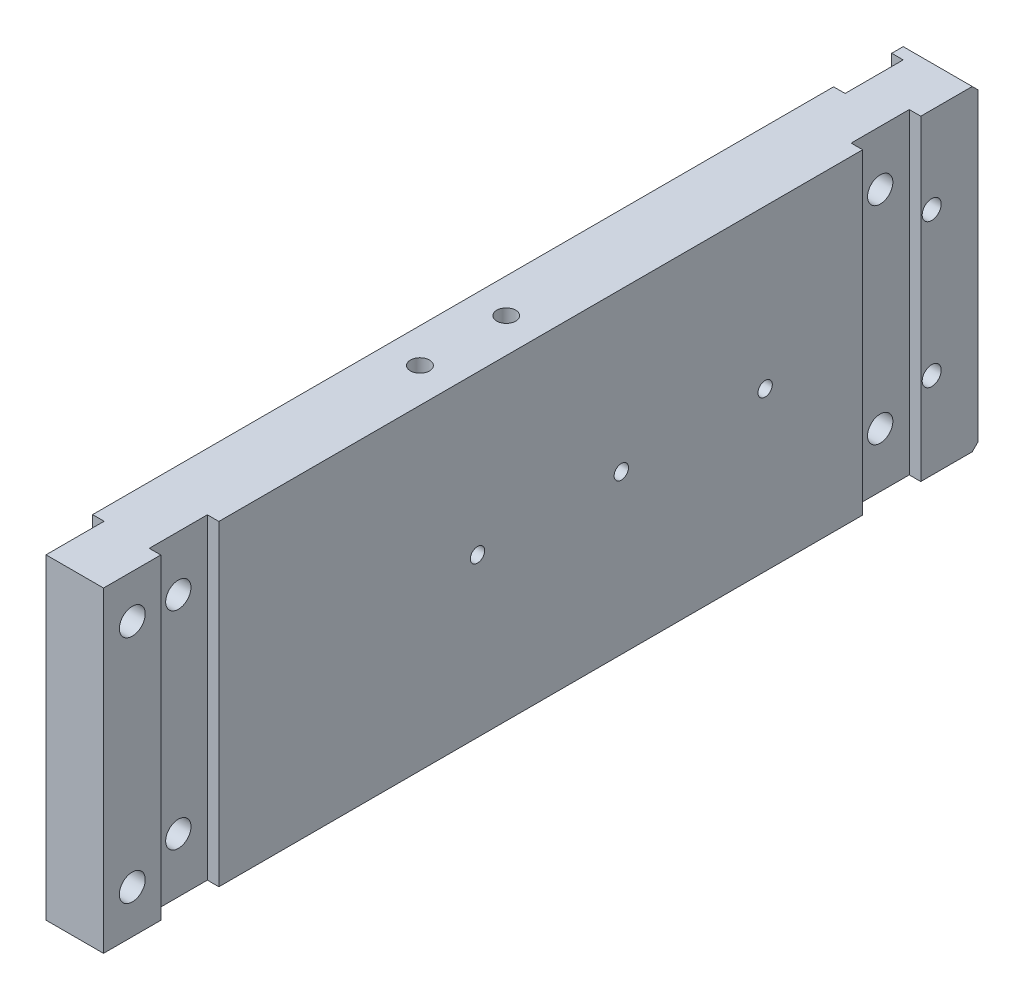
from build123d import *

# Parameters (mm, degrees)
SKETCH_1_W                  = 152
SKETCH_1_H                  = 55
EXTRUDE_1_DEPTH             = 12
SKETCH_2_W                  = 10.1
SKETCH_2_H                  = 67.741828953
CUT_EXTRUDE_1_DEPTH         = 2
SKETCH_3_W                  = 81
SKETCH_3_H                  = 12.05
CUT_EXTRUDE_2_DEPTH         = 1.5
SKETCH_4_R                  = 2
CUT_EXTRUDE_3_DEPTH         = 1.5
SKETCH_5_W                  = 2
SKETCH_5_H                  = 10.1
CUT_EXTRUDE_4_DEPTH         = 110
SKETCH_7_W                  = 4
SKETCH_7_H                  = 10.1
CUT_EXTRUDE_5_DEPTH         = 120
CHAMFER_1_SIZE              = 1
HOLE_WIZARD_M4_1_AT_2_COUNT = 2
HOLE_WIZARD_M4_1_AT_2_PITCH = 15
HOLE_WIZARD_5_0_5_2_D       = 5
HOLE_WIZARD_5_0_5_2_DEPTH   = 6
HOLE_WIZARD_5_0_5_2_TIP     = 1.502151548
HOLE_WIZARD_1_D             = 4.4
HOLE_WIZARD_1_CBORE_D       = 8
HOLE_WIZARD_1_CBORE_DEPTH   = 6
HOLE_WIZARD_M3_1_D          = 2.5
HOLE_WIZARD_M4_2_D          = 3.3
HOLE_WIZARD_M4_2_DEPTH      = 11.5
HOLE_WIZARD_M4_2_TIP        = 0.991420021
HOLE_WIZARD_M4_3_D          = 3.3
SKETCH_30_R                 = 2.25
CUT_EXTRUDE_6_DEPTH         = 25


with BuildPart() as part:
    # 草图1 → 凸台-拉伸1 (new body)
    with BuildSketch(Plane(origin=(0, 0, 0), x_dir=(0, 0, -1), z_dir=(1, 0, 0))):
        Rectangle(SKETCH_1_W, SKETCH_1_H)
    extrude(amount=EXTRUDE_1_DEPTH)

    # 草图2 → 切除-拉伸1 (cut)
    with BuildSketch(Plane(origin=(12, 0, 0), x_dir=(0, 0, -1), z_dir=(1, 0, 0))):
        with Locations((-61, -0.529795054)):
            Rectangle(SKETCH_2_W, SKETCH_2_H)
    cut_extrude_1 = extrude(amount=-CUT_EXTRUDE_1_DEPTH, mode=Mode.SUBTRACT)

    # 草图3 → 切除-拉伸2 (cut)
    with BuildSketch(Plane.ZY):
        with Locations((-13.5, 0)):
            Rectangle(SKETCH_3_W, SKETCH_3_H)
    extrude(amount=-CUT_EXTRUDE_2_DEPTH, mode=Mode.SUBTRACT)

    # 草图4 → 切除-拉伸3 (cut)
    with BuildSketch(Plane.ZY):
        with Locations((-54, 6.025)):
            Circle(SKETCH_4_R)
        with Locations((-54, -6.025)):
            Circle(SKETCH_4_R)
        with Locations((27, -6.025)):
            Circle(SKETCH_4_R)
        with Locations((27, 6.025)):
            Circle(SKETCH_4_R)
    extrude(amount=-CUT_EXTRUDE_3_DEPTH, mode=Mode.SUBTRACT)

    # 草图5 → 切除-拉伸4 (cut)
    with BuildSketch(Plane.XZ.offset(27.5)):
        with Locations((1, 70.95)):
            Rectangle(SKETCH_5_W, SKETCH_5_H)
    extrude(amount=-CUT_EXTRUDE_4_DEPTH, mode=Mode.SUBTRACT)

    # 草图7 → 切除-拉伸5 (cut)
    with BuildSketch(Plane(origin=(0, 27.5, 0), x_dir=(1, 0, 0), z_dir=(0, 1, 0))):
        with Locations((0, 67.95)):
            Rectangle(SKETCH_7_W, SKETCH_7_H)
    extrude(amount=-CUT_EXTRUDE_5_DEPTH, mode=Mode.SUBTRACT)

    # 倒角1
    chamfer_1_edges = [part.edges().sort_by_distance(p)[0] for p in [
        (6, -27.5, -76),
        (6, 27.5, -76),
    ]]
    chamfer(chamfer_1_edges, length=CHAMFER_1_SIZE)

    # 草图9 → M4 螺纹孔1 (revolve, cut)
    with BuildSketch(Plane(origin=(6, 27.5, 15), x_dir=(0, 0, 1), z_dir=(1, 0, 0))):
        Polygon((0, 0), (0, 11.091420021), (1.65, 10.1), (1.65, 0), align=None)
    hole_wizard_m4_1 = revolve(axis=Axis((6, 33.85, 15), (0, -1, 0)), mode=Mode.SUBTRACT)

    # M4 螺纹孔1 at 2: M4 螺纹孔1 ×2
    with Locations(*[(0, 0, -i * HOLE_WIZARD_M4_1_AT_2_PITCH) for i in range(1, HOLE_WIZARD_M4_1_AT_2_COUNT)]):
        add(hole_wizard_m4_1, mode=Mode.SUBTRACT)

    # 镜向1: M4 螺纹孔1 across plane
    add(hole_wizard_m4_1.mirror(Plane.ZX), mode=Mode.SUBTRACT)

    # 镜向1 copy 1 sketch → 镜向1 copy 1 (revolve, cut)
    with BuildSketch(Plane(origin=(6, -27.5, 0), x_dir=(0, 0, 1), z_dir=(1, 0, 0))):
        Polygon((0, 0), (0, -11.091420021), (1.65, -10.1), (1.65, 0), align=None)
    revolve(axis=Axis((6, -33.85, 0), (0, -1, 0)), mode=Mode.SUBTRACT)

    # Ø5.0 (5) 直径孔2
    with Locations(Plane.ZY.offset(-2)):
        with Locations((70.9, 12.5), (70.9, -12.5)):
            Hole(HOLE_WIZARD_5_0_5_2_D / 2, depth=HOLE_WIZARD_5_0_5_2_DEPTH)
            with Locations((0, 0, -(HOLE_WIZARD_5_0_5_2_DEPTH + HOLE_WIZARD_5_0_5_2_TIP / 2))):  # 118° drill point
                Cone(0, HOLE_WIZARD_5_0_5_2_D / 2, HOLE_WIZARD_5_0_5_2_TIP, mode=Mode.SUBTRACT)

    # 镜向2: 切除-拉伸1 across plane
    add(cut_extrude_1.mirror(Plane.XY), mode=Mode.SUBTRACT)

    # 打孔尺寸(%根据)内六角圆柱头螺钉的类型1 (through all)
    with Locations(Plane.ZY):
        with Locations((61, -18), (61, 18), (-61, 18), (-61, -18)):
            CounterBoreHole(HOLE_WIZARD_1_D / 2, HOLE_WIZARD_1_CBORE_D / 2, HOLE_WIZARD_1_CBORE_DEPTH)

    # M3 螺纹孔1 (through all)
    with Locations(Plane.ZY):
        with Locations((11, 0), (-14, 0), (-39, 0)):
            Hole(HOLE_WIZARD_M3_1_D / 2)

    # M4 螺纹孔2
    with Locations(Plane(origin=(0, -27.5, 0), x_dir=(-1, 0, 0), z_dir=(0, -1, 0))):
        with Locations((-6, 44.926), (-6, 59.926)):
            Hole(HOLE_WIZARD_M4_2_D / 2, depth=HOLE_WIZARD_M4_2_DEPTH)
            with Locations((0, 0, -(HOLE_WIZARD_M4_2_DEPTH + HOLE_WIZARD_M4_2_TIP / 2))):  # 118° drill point
                Cone(0, HOLE_WIZARD_M4_2_D / 2, HOLE_WIZARD_M4_2_TIP, mode=Mode.SUBTRACT)

    # M4 螺纹孔3 (through all)
    with Locations(Plane.ZY):
        with Locations((-67.95, 12.5), (-67.95, -12.5)):
            Hole(HOLE_WIZARD_M4_3_D / 2)

    # 草图30 → 切除-拉伸6 (cut)
    with BuildSketch(Plane(origin=(12, 0, 0), x_dir=(0, 0, -1), z_dir=(1, 0, 0))):
        with Locations((-71, 20)):
            Circle(SKETCH_30_R)
        with Locations((-71, -20)):
            Circle(SKETCH_30_R)
    extrude(amount=-CUT_EXTRUDE_6_DEPTH, mode=Mode.SUBTRACT)


solid = part.part
